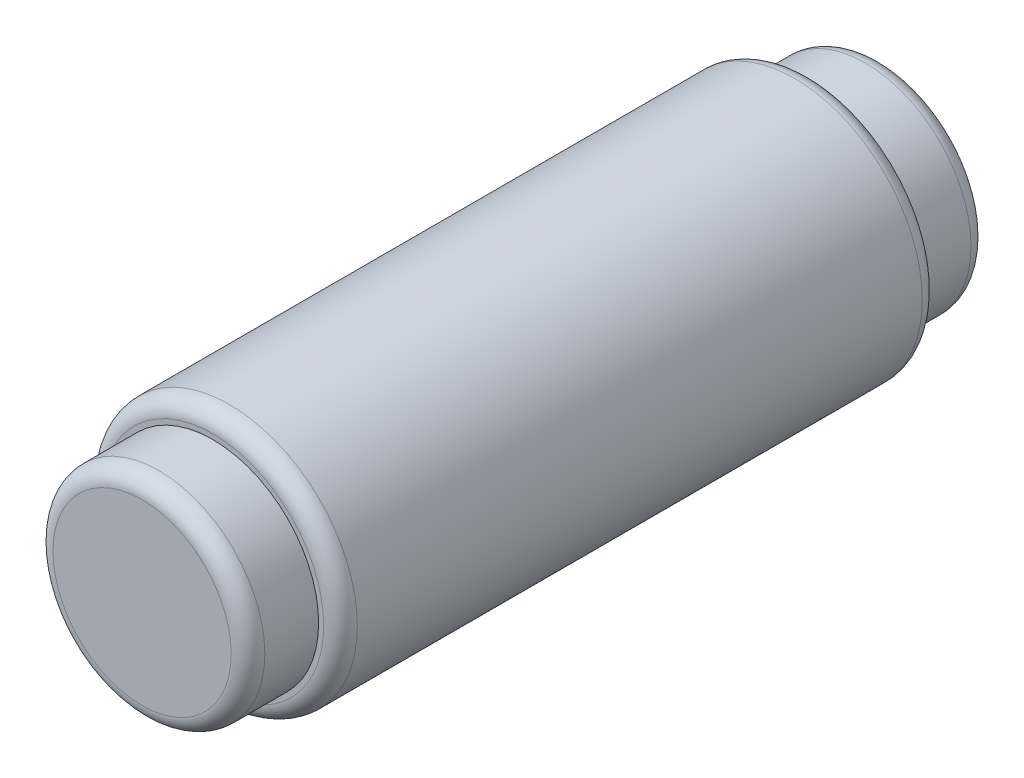
SolidWorks part; units mm, degrees
ref_plane "前视基准面" through (0, 0, 0) normal (0, 0, 1) x (1, 0, 0)
ref_plane "上视基准面" through (0, 0, 0) normal (0, 1, 0) x (1, 0, 0)
ref_plane "右视基准面" through (0, 0, 0) normal (1, 0, 0) x (0, 0, -1)
sketch "草图1" plane through (0, 0, 0) normal (0, 0, 1) x (1, 0, 0)
  circle A0 centre (0, 0) radius 38
  dimension "D1" = 76
extrude "凸台-拉伸1" add sketch "草图1" along normal mid plane 220
sketch "草图4" plane through (0, 0, 110) normal (0, 0, 1) x (1, 0, 0)
  circle A0 centre (0, 0) radius 31.5
  dimension "D1" = 63
extrude "切除-拉伸1" cut sketch "草图4" against normal blind 21 flip side to cut
sketch "草图5" plane through (0, 0, -110) normal (0, 0, -1) x (-1, 0, 0)
  circle A0 centre (0, 0) radius 31.5
  dimension "D1" = 63
extrude "切除-拉伸2" cut sketch "草图5" against normal blind 21 flip side to cut
fillet "圆角1" radius 5 4 edges at (-38, 0, -89) (38, 0, 89) (31.5, 0, 110) (-31.5, 0, -110)
sketch "草图2" plane through (0, 0, -110) normal (0, 0, -1) x (-1, 0, 0)
  circle A0 centre (0, 15.0142) radius 5.4789
  circle A1 centre (0, -16.3159) radius 5.5113
extrude "凸台-拉伸2" add sketch "草图2" along normal blind 2
